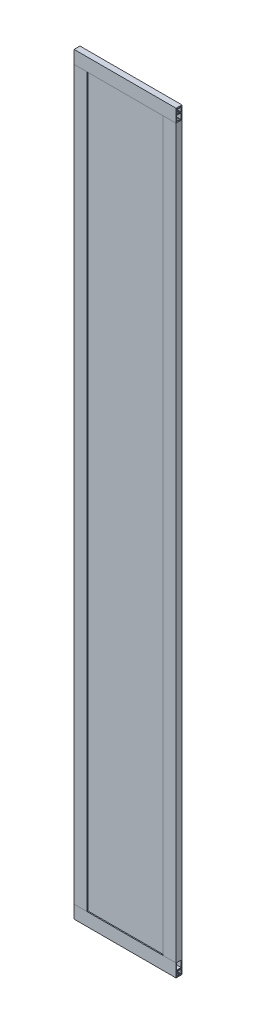
SolidWorks part; units mm, degrees
material "铝合金板 LF5"
ref_plane "前视基准面" through (0, 0, 0) normal (0, 0, 1) x (1, 0, 0)
ref_plane "上视基准面" through (0, 0, 0) normal (0, 1, 0) x (1, 0, 0)
ref_plane "右视基准面" through (0, 0, 0) normal (1, 0, 0) x (0, 0, -1)
sketch "草图1" plane through (0, 0, 0) normal (0, 0, 1) x (1, 0, 0)
  line L1 (-156.75, 1158.5) -> (156.75, 1158.5)
  line L2 (-156.75, 1158.5) -> (-156.75, -1158.5)
  line L3 (-156.75, -1158.5) -> (156.75, -1158.5)
  line L4 (156.75, 1158.5) -> (156.75, -1158.5)
  line L5 (-156.75, 1158.5) -> (156.75, -1158.5) construction
  line L6 (-156.75, -1158.5) -> (156.75, 1158.5) construction
  point P0 (0, 0)
other "自定义 玻璃外框(1)"
ref_plane "基准面4" through (-156.75, 1158.5, 0) normal (1, 0, 0) x (0, 0, -1)
sketch "Sketch1" plane through (-156.75, 1158.5, 0) normal (1, 0, 0) x (0, 0, -1)
  line L8 (-1.3416, -18) -> (1.3416, -18)
  line L9 (2.6401, -18) -> (7, -18)
  line L10 (7, -18) -> (7, -3)
  line L11 (7, -3) -> (2.6401, -3)
  line L12 (1.3416, -3) -> (-1.3416, -3)
  line L13 (-2.6401, -3) -> (-7, -3)
  line L14 (-7, -3) -> (-7, -18)
  line L15 (-7, -18) -> (-2.6401, -18)
  line L17 (7, -38.5) -> (5.9, -38.5)
  line L18 (5.9, -38.5) -> (5.9, -40)
  line L19 (5.9, -40) -> (7, -40)
  line L20 (7, -40) -> (9, -40)
  line L21 (9, -40) -> (9, 0)
  line L22 (9, 0) -> (-9, 0)
  line L23 (-9, 0) -> (-9, -40)
  line L24 (-9, -40) -> (-7, -40)
  line L25 (-7, -40) -> (-5.9, -40)
  line L26 (-5.9, -40) -> (-5.9, -38.5)
  line L27 (-5.9, -38.5) -> (-7, -38.5)
  line L28 (-7, -38.5) -> (-7, -20)
  line L29 (-7, -20) -> (7, -20)
  line L30 (7, -20) -> (7, -38.5)
  arc A0 (2.0506, -14.7494) -> (1.2728, -15.5272) centre (1.6617, -15.1383) ccw
  arc A1 (2.6401, -18) -> (2.0506, -14.7494) centre (0, -16.8) ccw
  arc A2 (2.0506, -6.2506) -> (2.6401, -3) centre (0, -4.2) ccw
  arc A3 (1.2728, -5.4728) -> (2.0506, -6.2506) centre (1.6617, -5.8617) ccw
  arc A4 (1.2728, -5.4728) -> (1.3416, -3) centre (0, -4.2) ccw
  arc A5 (-1.3416, -3) -> (-1.2728, -5.4728) centre (0, -4.2) ccw
  arc A6 (-2.0506, -6.2506) -> (-1.2728, -5.4728) centre (-1.6617, -5.8617) ccw
  arc A7 (-2.6401, -3) -> (-2.0506, -6.2506) centre (0, -4.2) ccw
  arc A8 (-2.0506, -14.7494) -> (-2.6401, -18) centre (0, -16.8) ccw
  arc A9 (-1.2728, -15.5272) -> (-2.0506, -14.7494) centre (-1.6617, -15.1383) ccw
  arc A10 (-1.2728, -15.5272) -> (-1.3416, -18) centre (0, -16.8) ccw
  arc A11 (1.3416, -18) -> (1.2728, -15.5272) centre (0, -16.8) ccw
  point P0 (0, 0)
sketch "草图2" plane through (0, 0, 9) normal (0, 0, 1) x (1, 0, 0)
  line L0 (116.75, 1118.5) -> (-116.75, -1118.5) construction
  line L1 (156.75, 1158.5) -> (-156.75, 1158.5) construction
  line L2 (-133.75, 1135.5) -> (133.75, 1135.5)
  line L3 (-133.75, 1135.5) -> (-133.75, -1135.5)
  line L4 (-133.75, -1135.5) -> (133.75, -1135.5)
  line L5 (133.75, 1135.5) -> (133.75, -1135.5)
  line L6 (-133.75, 1135.5) -> (133.75, -1135.5) construction
  line L7 (-133.75, -1135.5) -> (133.75, 1135.5) construction
  line L8 (156.75, -1118.5) -> (156.75, 1118.5) construction
  point P4 (0, 0)
  dimension "D1" = 23
  dimension "D2" = 23
  dimension "D3" = 267.5
  dimension "D4" = 2271
extrude "凸台-拉伸1" add sketch "草图2" against normal blind 10 from offset 3.1 separate body offset against normal yes
equation "\"A\" =1195"
equation "\"B\" =1155"
equation "\"CH\" = 2300"
equation "\"OP\" =750"
equation "\"OPH\" = 2100"
equation "\"QB\" = 50"
equation "\"DK\" = 40"
equation "\"WCOP\" =0"
equation "\"HCOP\" =4"
equation "\"FJ\" = 2"
equation "\"DH\" = 16"
equation "\"LG\" = 1"
equation "\"DD\" = 2"
equation "\"C\" =545"
equation "\"PX\" =-75"
equation "\"LZ\" = 350"
equation "\"LJ\" = 1158"
equation "\"LLK\" = 310"
equation "\"FS\" = 0"
equation "\"后玻璃框（纵）\"= \"CH\" + \"DH\" + 1"
equation "\"后玻璃框（横）\"= 0'见轿厢"
equation "\"D2@草图1\"=\"后玻璃框（纵）\""
